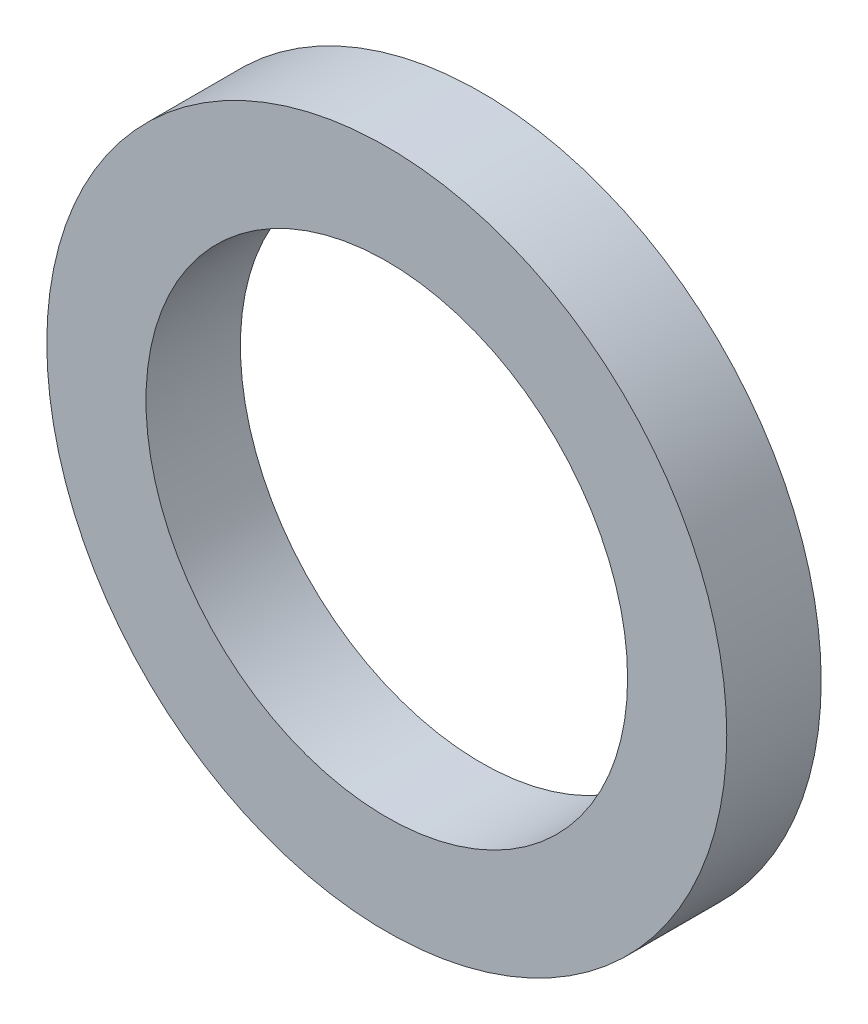
from build123d import *

# Parameters (mm, degrees)
SKETCH1_R           = 18
SKETCH1_R_2         = 12.75
BOSS_EXTRUDE1_DEPTH = 5


with BuildPart() as part:
    # Sketch1 → Boss-Extrude1 (new body)
    with BuildSketch(Plane.XY):
        Circle(SKETCH1_R)
        Circle(SKETCH1_R_2, mode=Mode.SUBTRACT)
    extrude(amount=BOSS_EXTRUDE1_DEPTH)


solid = part.part
